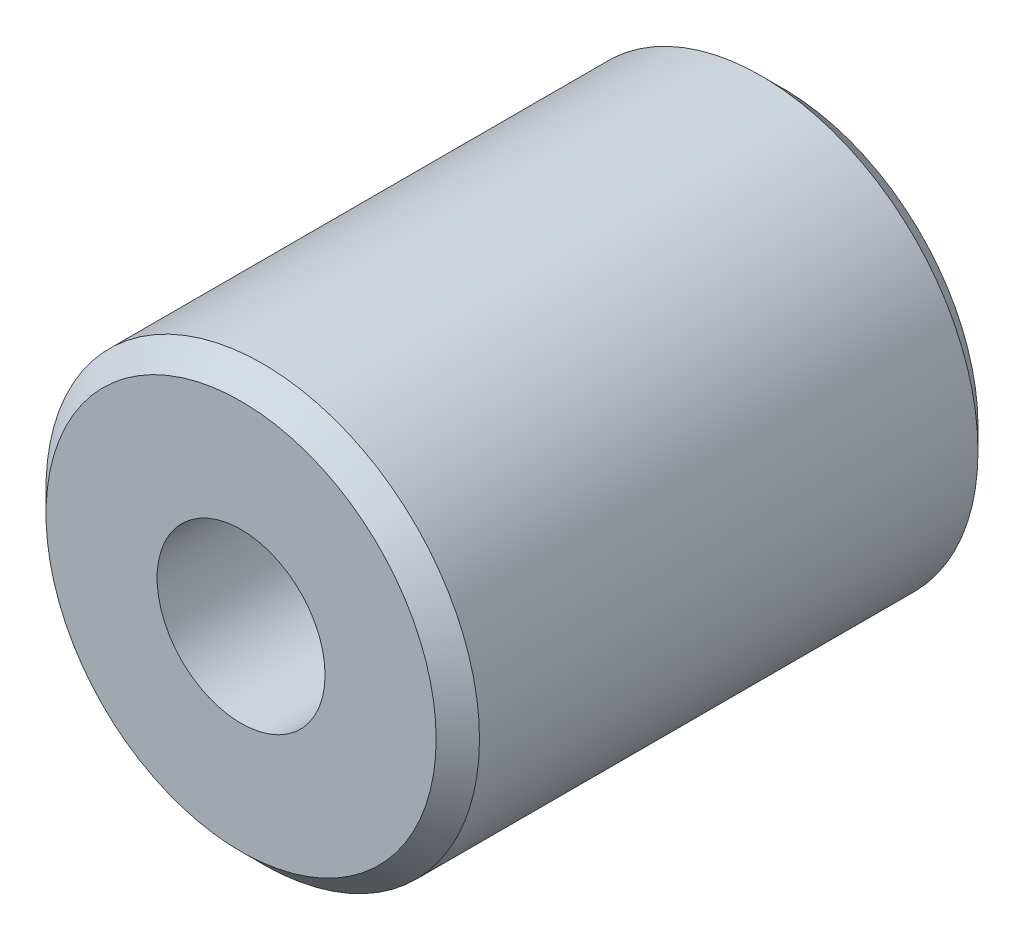
from build123d import *

# Parameters (mm, degrees)
SKETCH1_R           = 20
BOSS_EXTRUDE1_DEPTH = 25
CHAMFER1_SIZE       = 2
M18_TAPPED_HOLE1_D  = 15.5


with BuildPart() as part:
    # Sketch1 → Boss-Extrude1 (new, symmetric)
    with BuildSketch(Plane.XY):
        Circle(SKETCH1_R)
    extrude(amount=BOSS_EXTRUDE1_DEPTH, both=True)

    # Chamfer1
    chamfer1_edges = [part.edges().sort_by_distance(p)[0] for p in [
        (-20, 0, -25),
        (-20, 0, 25),
    ]]
    chamfer(chamfer1_edges, length=CHAMFER1_SIZE)

    # M18 Tapped Hole1 (through all)
    with Locations(Plane.XY.offset(25)):
        with Locations((0, 0)):
            Hole(M18_TAPPED_HOLE1_D / 2)


solid = part.part
